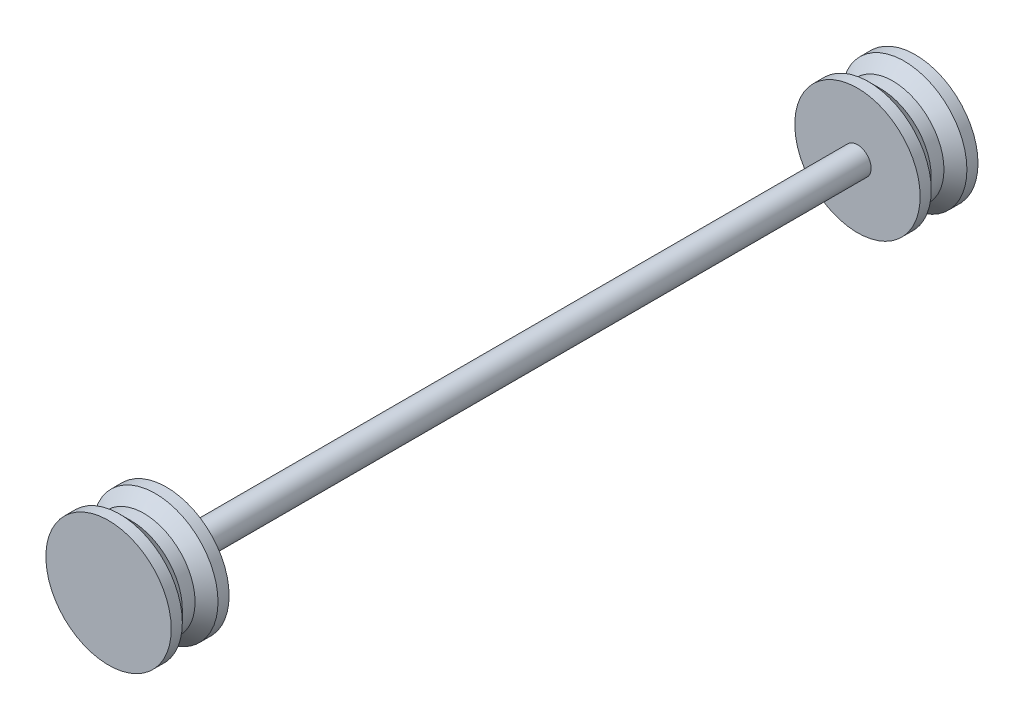
SolidWorks part; units mm, degrees
ref_plane "Front Plane" through (0, 0, 0) normal (0, 0, 1) x (1, 0, 0)
ref_plane "Top Plane" through (0, 0, 0) normal (0, 1, 0) x (1, 0, 0)
ref_plane "Right Plane" through (0, 0, 0) normal (1, 0, 0) x (0, 0, -1)
other "Configuration Table"
sketch "Sketch1" plane through (0, 0, 0) normal (0, 0, 1) x (1, 0, 0)
  circle A0 centre (-29.7913, -6.2198) radius 1.1795
extrude "Boss-Extrude1" add sketch "Sketch1" against normal up to surface (59.7318 mm away)
sketch "Sketch2" plane through (0, 0, 0) normal (0, 0, 1) x (1, 0, 0)
  circle A0 centre (-29.7913, -6.2198) radius 5.4178
extrude "Boss-Extrude2" add sketch "Sketch2" along normal blind 5
ref_axis "Axis1" through (-29.7913, -6.2198, 5) along (0, 0, -1)
ref_plane "Plane1" through (0, -6.2198, 0) normal (0, 1, 0) x (0, 0, -1)
ref_plane "Plane2" through (0, 0, -29.8659) normal (0, 0, 1) x (1, 0, 0)
mirror "Mirror1" about plane through (0, 0, -29.8659) normal (0, 0, 1) of "Boss-Extrude2"
sketch "Sketch4" plane through (0, -6.2198, 0) normal (0, 1, 0) x (0, 0, -1)
  line L0 (-4.0421, 35.2091) -> (-3.0506, 34.2176)
  line L1 (0, 35.2091) -> (-5, 35.2091) construction
  line L2 (-3.0506, 34.2176) -> (-1.9494, 34.2176)
  line L4 (-0.9579, 35.2091) -> (-4.0421, 35.2091)
  line L5 (-0.9579, 35.2091) -> (-1.9494, 34.2176)
  line L6 (60.6897, 35.2091) -> (61.6812, 34.2176)
  line L7 (61.6812, 34.2176) -> (62.7824, 34.2176)
  line L8 (63.7739, 35.2091) -> (60.6897, 35.2091)
  line L9 (63.7739, 35.2091) -> (62.7824, 34.2176)
revolve "Cut-Revolve2" cut sketch "Sketch4" angle 360 about axis through (-29.7913, -6.2198, 5) along (0, 0, -1)
